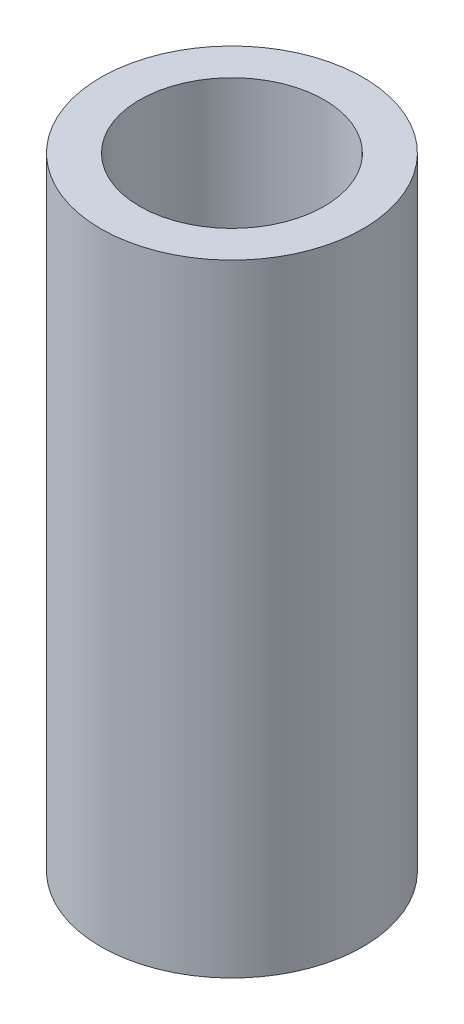
SolidWorks part; units mm, degrees
ref_plane "Front Plane" through (0, 0, 0) normal (0, 0, 1) x (1, 0, 0)
ref_plane "Top Plane" through (0, 0, 0) normal (0, 1, 0) x (1, 0, 0)
ref_plane "Right Plane" through (0, 0, 0) normal (1, 0, 0) x (0, 0, -1)
sketch "Sketch1" plane through (0, 0, 0) normal (0, 1, 0) x (1, 0, 0)
  circle A0 centre (0, 0) radius 9.5
  circle A1 centre (0, 0) radius 13.5
  dimension "D1" = 19
  dimension "D2" = 27
extrude "Extrude1" add sketch "Sketch1" along normal blind 64
